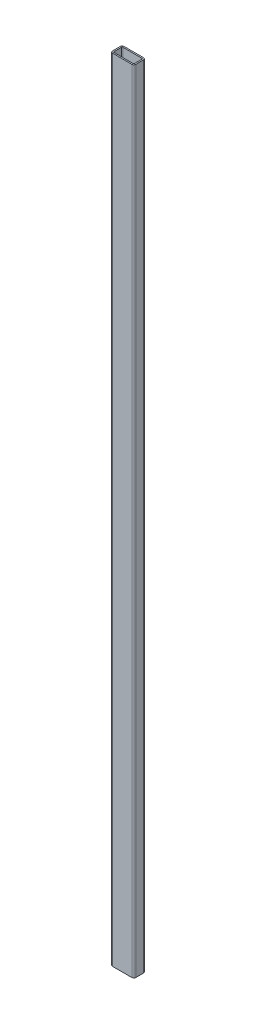
from build123d import *

# Parameters (mm, degrees)
BOSS_EXTRUDE1_DEPTH = 1360


with BuildPart() as part:
    # Sketch1 → Boss-Extrude1 (new body)
    with BuildSketch(Plane(origin=(0, 0, 0), x_dir=(1, 0, 0), z_dir=(0, 1, 0))):
        with BuildLine():
            Line((-16.55, -10), (16.55, -10))
            ThreePointArc((16.55, -10), (18.989518395, -8.989518395), (20, -6.55))
            Line((20, -6.55), (20, 6.55))
            ThreePointArc((20, 6.55), (18.989518395, 8.989518395), (16.55, 10))
            Line((16.55, 10), (-16.55, 10))
            ThreePointArc((-16.55, 10), (-18.989518395, 8.989518395), (-20, 6.55))
            Line((-20, 6.55), (-20, -6.55))
            ThreePointArc((-20, -6.55), (-18.989518395, -8.989518395), (-16.55, -10))
        make_face()
        with BuildLine():
            Line((-16.55, -7.7), (16.55, -7.7))
            ThreePointArc((16.55, -7.7), (17.363172798, -7.363172798), (17.7, -6.55))
            Line((17.7, -6.55), (17.7, 6.55))
            ThreePointArc((17.7, 6.55), (17.363172798, 7.363172798), (16.55, 7.7))
            Line((16.55, 7.7), (-16.55, 7.7))
            ThreePointArc((-16.55, 7.7), (-17.363172798, 7.363172798), (-17.7, 6.55))
            Line((-17.7, 6.55), (-17.7, -6.55))
            ThreePointArc((-17.7, -6.55), (-17.363172798, -7.363172798), (-16.55, -7.7))
        make_face(mode=Mode.SUBTRACT)
    extrude(amount=BOSS_EXTRUDE1_DEPTH)


solid = part.part
